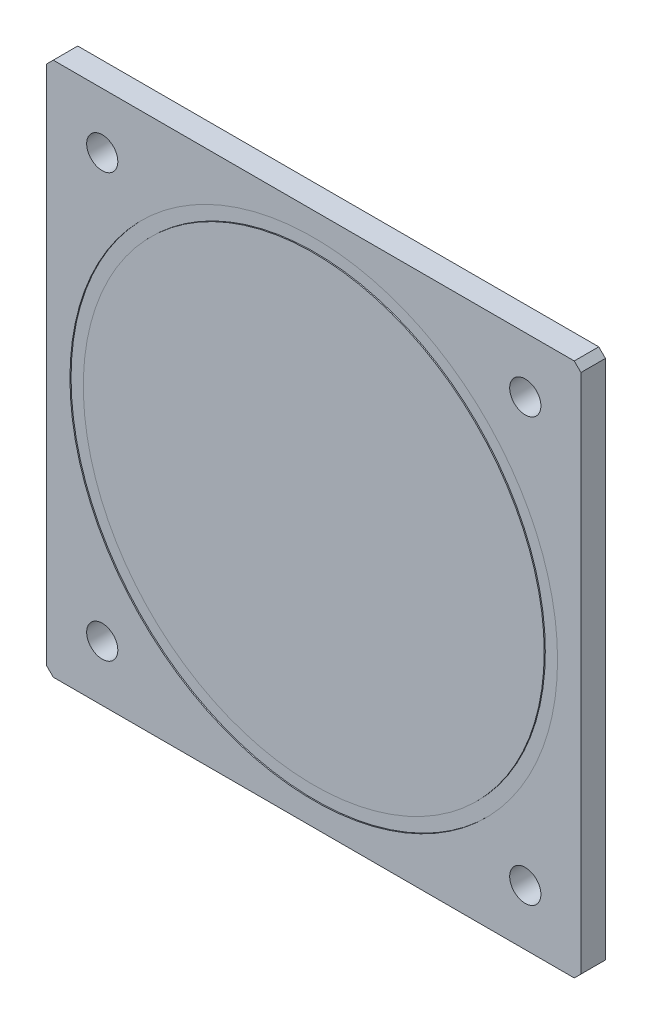
SolidWorks part; units mm, degrees
ref_plane "Front Plane" through (0, 0, 0) normal (0, 0, 1) x (1, 0, 0)
ref_plane "Top Plane" through (0, 0, 0) normal (0, 1, 0) x (1, 0, 0)
ref_plane "Right Plane" through (0, 0, 0) normal (1, 0, 0) x (0, 0, -1)
sketch "Sketch1" plane through (0, 0, 0) normal (0, 0, 1) x (1, 0, 0)
  line L1 (120, 120) -> (-120, 120)
  line L2 (120, 120) -> (120, -120)
  line L3 (120, -120) -> (-120, -120)
  line L4 (-120, 120) -> (-120, -120)
  line L5 (120, 120) -> (-120, -120) construction
  line L6 (120, -120) -> (-120, 120) construction
  point P0 (0, 0)
  dimension "D1" = 240
  dimension "D2" = 240
extrude "Boss-Extrude1" add sketch "Sketch1" along normal blind 11
sketch "Sketch2" plane through (0, 0, 11) normal (0, 0, 1) x (1, 0, 0)
  circle A0 centre (0, 0) radius 103.5
  circle A1 centre (0, 0) radius 109.5
  dimension "D1" = 219
  dimension "D2" = 207
extrude "Cut-Extrude1" cut sketch "Sketch2" against normal blind 0.5
sketch "Sketch3" plane through (0, 0, 11) normal (0, 0, 1) x (1, 0, 0)
  line L1 (95, 95) -> (-95, 95) construction
  line L2 (95, 95) -> (95, -95) construction
  line L3 (95, -95) -> (-95, -95) construction
  line L4 (-95, 95) -> (-95, -95) construction
  line L5 (95, 95) -> (-95, -95) construction
  line L6 (95, -95) -> (-95, 95) construction
  circle A0 centre (-95, 95) radius 7
  circle A1 centre (95, 95) radius 7
  circle A2 centre (95, -95) radius 7
  circle A3 centre (-95, -95) radius 7
  point P0 (0, 0)
  dimension "D3" = 14
  dimension "D1" = 190
  dimension "D2" = 190
extrude "Cut-Extrude2" cut sketch "Sketch3" against normal blind 59
chamfer "Chamfer1" distance 3 angle 45 4 edges at (-120, -120, 5.5) (120, -120, 5.5) (120, 120, 5.5) (-120, 120, 5.5)
